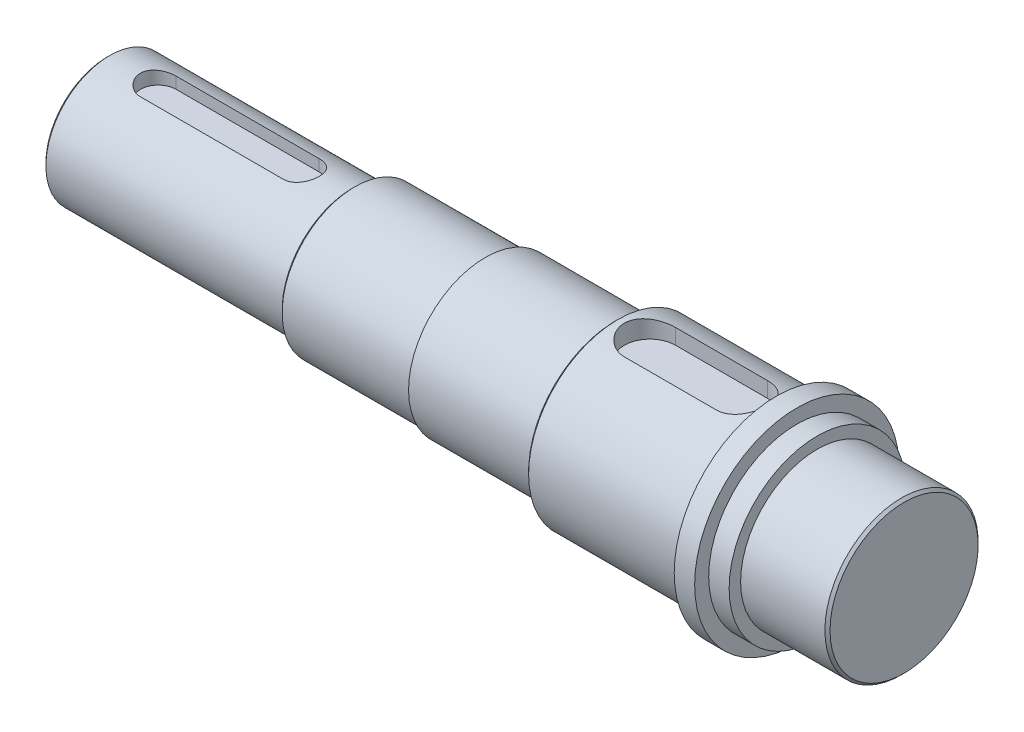
SolidWorks part; units mm, degrees
material "1.0503 (C45)"
ref_plane "Front Plane" through (0, 0, 0) normal (0, 0, 1) x (1, 0, 0)
ref_plane "Top Plane" through (0, 0, 0) normal (0, 1, 0) x (1, 0, 0)
ref_plane "Right Plane" through (0, 0, 0) normal (1, 0, 0) x (0, 0, -1)
sketch "Sketch1" plane through (0, 0, 0) normal (0, 0, 1) x (1, 0, 0)
  line L0 (0, 0) -> (0, 25)
  line L1 (0, 25) -> (96, 25)
  line L2 (96, 25) -> (96, 28.5)
  line L3 (96, 28.5) -> (148, 28.5)
  line L4 (148, 28.5) -> (148, 30)
  line L5 (148, 30) -> (199, 30)
  line L6 (199, 30) -> (199, 35)
  line L7 (199, 35) -> (262, 35)
  line L8 (262, 35) -> (262, 40)
  line L9 (262, 40) -> (270, 40)
  line L10 (270, 40) -> (270, 34.5)
  line L11 (270, 34.5) -> (278, 34.5)
  line L12 (278, 34.5) -> (278, 30)
  line L13 (278, 30) -> (312, 30)
  line L14 (312, 30) -> (312, 0)
  line L15 (0, 0) -> (340.5721, 0) construction
  line L16 (0, 0) -> (312, 0)
  point P17 (274, 34.5)
  dimension "D1" = 25
  dimension "D2" = 96
  dimension "D3" = 28.5
  dimension "D4" = 52
  dimension "D5" = 30
  dimension "D6" = 51
  dimension "D7" = 35
  dimension "D8" = 63
  dimension "D9" = 40
  dimension "D10" = 8
  dimension "D11" = 34.5
  dimension "D12" = 30
  dimension "D13" = 34
  dimension "D14" = 8
revolve "Revolve3" add sketch "Sketch1" angle 360 about L15
chamfer "Chamfer1" distance 1 angle 45 1 edges at (0, 0, 25)
chamfer "Chamfer2" distance 1 angle 45 1 edges at (312, 0, 30)
fillet "Fillet1" radius 0.5 2 edges at (148, 0, 28.5) (96, 0, 25)
chamfer "Chamfer3" distance 1 angle 45 1 edges at (199, 0, 35)
chamfer "Chamfer4" distance 1 angle 45 1 edges at (96, 0, 28.5)
fillet "Fillet2" radius 0.5 1 edges at (199, 0, 30)
sketch "Sketch2" plane through (0, 0, 0) normal (0, 1, 0) x (1, 0, 0)
  line L0 (20, 0) -> (76, 0) construction
  line L1 (20, 7) -> (76, 7)
  line L2 (20, -7) -> (76, -7)
  line L3 (0, 24) -> (0, -24) construction
  arc A0 (20, 7) -> (20, -7) centre (20, 0) ccw
  arc A1 (76, -7) -> (76, 7) centre (76, 0) ccw
  point P3 (48, 0)
  dimension "D1" = 14
  dimension "D2" = 48
  dimension "D3" = 56
extrude "Cut-Extrude1" cut sketch "Sketch2" along normal blind 20 from offset 19.5
sketch "Sketch3" plane through (0, 0, 0) normal (0, 1, 0) x (1, 0, 0)
  line L0 (212.5, 0) -> (248.5, 0) construction
  line L1 (212.5, 10) -> (248.5, 10)
  line L2 (212.5, -10) -> (248.5, -10)
  line L3 (262, 35) -> (262, -35) construction
  arc A0 (212.5, 10) -> (212.5, -10) centre (212.5, 0) ccw
  arc A1 (248.5, -10) -> (248.5, 10) centre (248.5, 0) ccw
  point P3 (230.5, 0)
  dimension "D1" = 20
  dimension "D2" = 36
  dimension "D3" = 31.5
extrude "Cut-Extrude2" cut sketch "Sketch3" along normal blind 20 from offset 27.5
